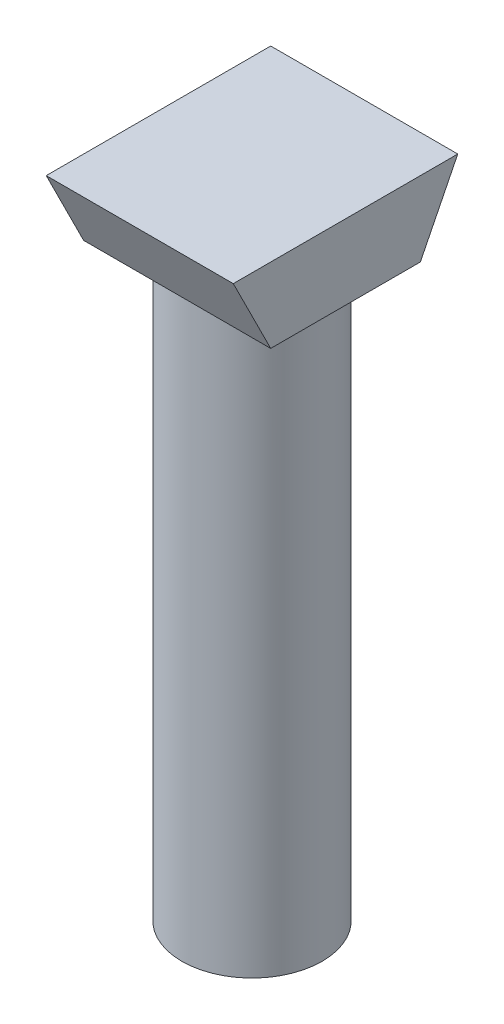
SolidWorks part; units mm, degrees
material "Q235-A"
ref_plane "Front Plane" through (0, 0, 0) normal (0, 0, 1) x (1, 0, 0)
ref_plane "Top Plane" through (0, 0, 0) normal (0, 1, 0) x (1, 0, 0)
ref_plane "Right Plane" through (0, 0, 0) normal (1, 0, 0) x (0, 0, -1)
sketch "Sketch1" plane through (0, 0, 0) normal (1, 0, 0) x (0, 0, -1)
  line L1 (24, -8) -> (-24, -8)
  line L2 (24, -8) -> (24, 8)
  line L3 (24, 8) -> (-24, 8)
  line L4 (-24, -8) -> (-24, 8)
  line L5 (24, -8) -> (-24, 8) construction
  line L6 (24, 8) -> (-24, -8) construction
  point P0 (0, 0)
  dimension "D1" = 48
  dimension "D2" = 16
extrude "Boss-Extrude1" add sketch "Sketch1" along normal mid plane 40
sketch "Sketch2" plane through (0, 0, 0) normal (1, 0, 0) x (0, 0, -1)
  line L0 (-24, 8) -> (-16, -8)
  line L1 (-24, -8) -> (24, -8) construction
  line L2 (-16, -8) -> (-24, -8)
  line L3 (-24, -8) -> (-24, 8)
  line L4 (0, 0) -> (0, -32.9014) construction
  line L5 (24, 8) -> (24, -8)
  line L6 (24, -8) -> (16, -8)
  line L7 (16, -8) -> (24, 8)
  dimension "D1" = 32
extrude "Cut-Extrude1" cut sketch "Sketch2" against normal through all both and the other way through all
sketch "Sketch3" plane through (0, -8, 0) normal (0, -1, 0) x (1, 0, 0)
  circle A0 centre (0, 0) radius 15
  dimension "D1" = 30
extrude "Boss-Extrude2" add sketch "Sketch3" along normal blind 124
